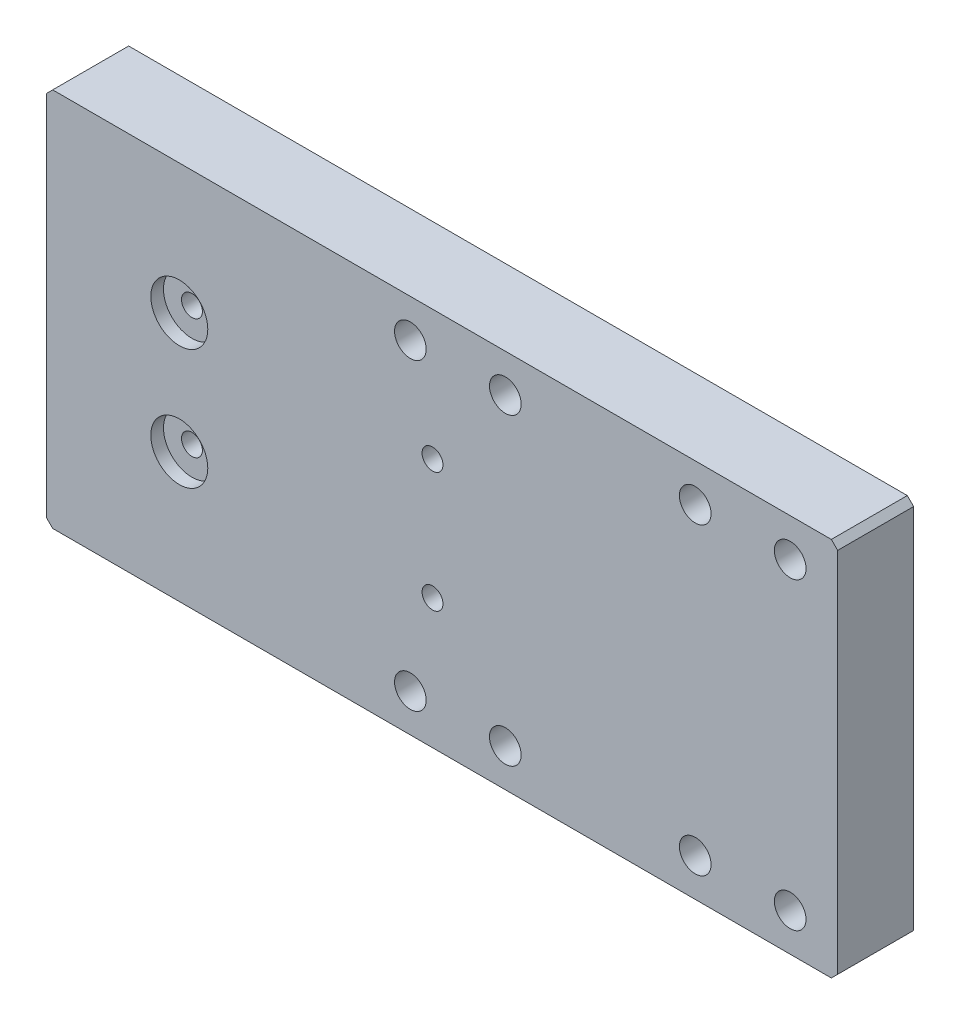
SolidWorks part; units mm, degrees
material "AL6061"
ref_plane "Front Plane" through (0, 0, 0) normal (0, 0, 1) x (1, 0, 0)
ref_plane "Top Plane" through (0, 0, 0) normal (0, 1, 0) x (1, 0, 0)
ref_plane "Right Plane" through (0, 0, 0) normal (1, 0, 0) x (0, 0, -1)
sketch "Sketch1" plane through (0, 0, 0) normal (0, 0, 1) x (1, 0, 0)
  line L1 (-62.5, 30) -> (62.5, 30)
  line L2 (-62.5, 30) -> (-62.5, -30)
  line L3 (-62.5, -30) -> (62.5, -30)
  line L4 (62.5, 30) -> (62.5, -30)
  line L5 (-62.5, 30) -> (62.5, -30) construction
  line L6 (-62.5, -30) -> (62.5, 30) construction
  point P0 (0, 0)
  dimension "D1" = 60
  dimension "D2" = 125
extrude "Boss-Extrude1" add sketch "Sketch1" along normal mid plane 12
hole_wizard "M6 Tapped Hole1" positions "Sketch4" profile "Sketch5" tap size "M6" standard "ISO" end condition through all
sketch "Sketch4" plane through (0, 0, -6) normal (0, 0, -1) x (-1, 0, 0)
  point P0 (5, 24)
  point P3 (5, -24)
  point P6 (-55, -24)
  point P9 (-55, 24)
sketch "Sketch5" plane through (-5, 24, -6) normal (1, 0, 0) x (0, 1, 0)
  line L0 (0, 0) -> (0, 12)
  line L1 (0, 12) -> (2.5, 12)
  line L2 (2.5, 12) -> (2.5, 0)
  line L5 (2.5, 0) -> (0, 0)
  line L11 (0, -6.35) -> (0, 107.95) construction
  dimension "通孔螺纹孔钻头直径" = 5
  dimension "通孔螺纹孔钻头深度" = 12
cosmetic thread "Cosmetic Thread1" parameters "D2"=6
cosmetic thread "Cosmetic Thread2" parameters "D2"=6
cosmetic thread "Cosmetic Thread3" parameters "D2"=6
cosmetic thread "Cosmetic Thread4" parameters "D2"=6
hole_wizard "M4 Tapped Hole1" positions "Sketch6" profile "Sketch7" tap size "M4" standard "ISO" end condition through all
sketch "Sketch6" plane through (0, 0, 6) normal (0, 0, 1) x (1, 0, 0)
  point P0 (-1.5, 9.5)
  point P3 (-1.5, -9.5)
  point P6 (-41.5, -9.5)
  point P9 (-41.5, 9.5)
sketch "Sketch7" plane through (-1.5, 9.5, 6) normal (1, 0, 0) x (0, -1, 0)
  line L0 (0, 0) -> (0, 12)
  line L1 (0, 12) -> (1.65, 12)
  line L2 (1.65, 12) -> (1.65, 0)
  line L5 (1.65, 0) -> (0, 0)
  line L11 (0, -6.35) -> (0, 107.95) construction
  dimension "通孔螺纹孔钻头直径" = 3.3
  dimension "通孔螺纹孔钻头深度" = 12
cosmetic thread "Cosmetic Thread5" parameters "D2"=4
cosmetic thread "Cosmetic Thread6" parameters "D2"=4
cosmetic thread "Cosmetic Thread7" parameters "D2"=4
cosmetic thread "Cosmetic Thread8" parameters "D2"=4
sketch "Sketch8" plane through (0, 0, 6) normal (0, 0, 1) x (1, 0, 0)
  circle A0 centre (-41.5, 9.5) radius 4.5
  circle A1 centre (-41.5, -9.5) radius 4.5
  dimension "D1" = 9
extrude "Cut-Extrude1" cut sketch "Sketch8" against normal blind 2
hole_wizard "Blind Pin Hole1 (size mm)" positions "Sketch9" profile "Sketch10" hole size "Ø5.0" standard "ISO" end condition through all
sketch "Sketch9" plane through (0, 0, 6) normal (0, 0, 1) x (1, 0, 0)
  point P0 (10, 24)
  point P3 (40, 24)
  point P6 (10, -24)
  point P9 (40, -24)
sketch "Sketch10" plane through (10, 24, 6) normal (1, 0, 0) x (0, -1, 0)
  line L0 (0, 0) -> (0, 12)
  line L1 (0, 12) -> (2.5, 12)
  line L2 (2.5, 12) -> (2.5, 0)
  line L5 (2.5, 0) -> (0, 0)
  line L11 (0, -6.35) -> (0, 107.95) construction
  dimension "通孔孔直径" = 5
  dimension "通孔孔深度" = 12
chamfer "Chamfer1" distance 1 angle 45 4 edges at (62.5, -30, 0) (62.5, 30, 0) (-62.5, 30, 0) (-62.5, -30, 0)
